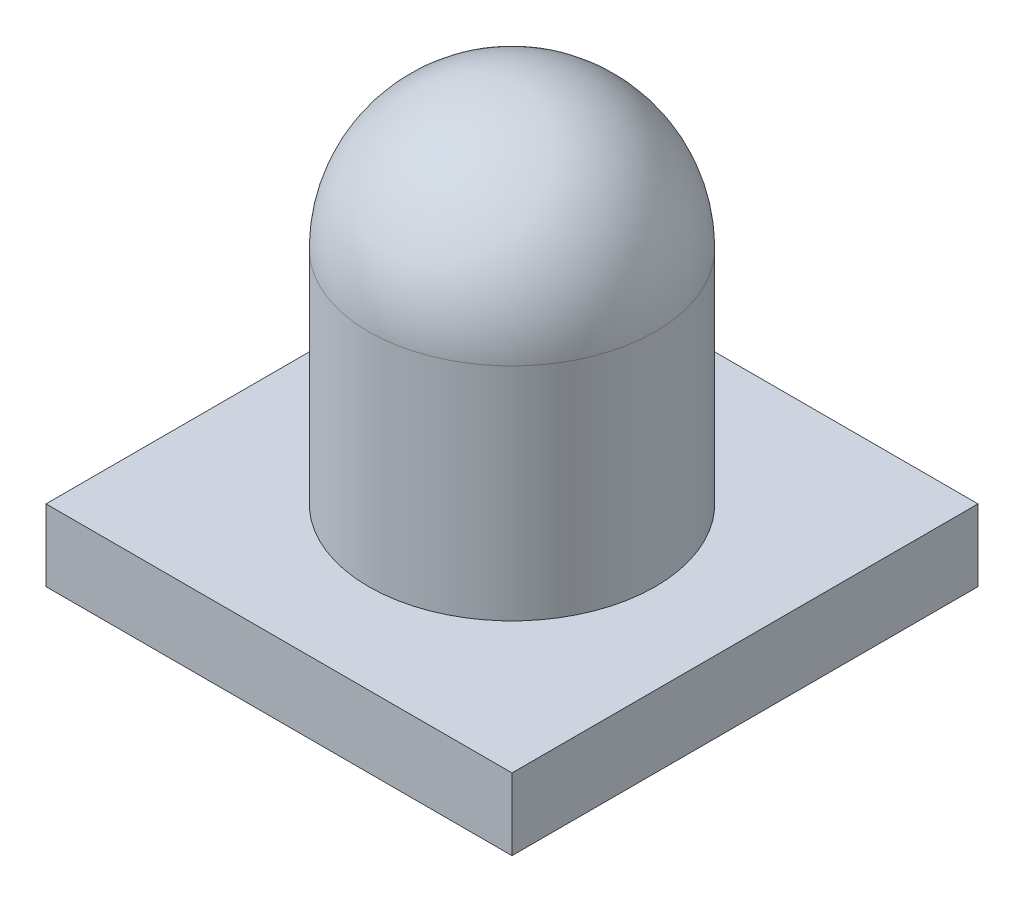
SolidWorks part; units mm, degrees
ref_plane "Front Plane" through (0, 0, 0) normal (0, 0, 1) x (1, 0, 0)
ref_plane "Top Plane" through (0, 0, 0) normal (0, 1, 0) x (1, 0, 0)
ref_plane "Right Plane" through (0, 0, 0) normal (1, 0, 0) x (0, 0, -1)
sketch "Sketch1" plane through (0, 0, 0) normal (0, 1, 0) x (1, 0, 0)
  line L1 (-32.5, -32.5) -> (32.5, -32.5)
  line L2 (-32.5, -32.5) -> (-32.5, 32.5)
  line L3 (-32.5, 32.5) -> (32.5, 32.5)
  line L4 (32.5, -32.5) -> (32.5, 32.5)
  line L5 (-32.5, -32.5) -> (32.5, 32.5) construction
  line L6 (-32.5, 32.5) -> (32.5, -32.5) construction
  point P0 (0, 0)
  dimension "D1" = 65
  dimension "D2" = 65
extrude "Boss-Extrude1" add sketch "Sketch1" along normal blind 10
sketch "Sketch2" plane through (0, 10, 0) normal (0, 1, 0) x (1, 0, 0)
  circle A0 centre (0, 0) radius 20
  dimension "D1" = 40
extrude "Boss-Extrude2" add sketch "Sketch2" along normal blind 50.8
fillet "Fillet1" radius 20 1 edges at (0, 60.8, 20)
sketch "Sketch3" plane through (0, 0, 0) normal (0, -1, 0) x (1, 0, 0)
  line L1 (-24, -18) -> (24, -18) construction
  line L2 (-24, -18) -> (-24, 18) construction
  line L3 (-24, 18) -> (24, 18) construction
  line L4 (24, -18) -> (24, 18) construction
  line L5 (-24, -18) -> (24, 18) construction
  line L6 (-24, 18) -> (24, -18) construction
  circle A0 centre (24, 18) radius 1.5
  circle A1 centre (-24, 18) radius 1.5
  circle A2 centre (-24, -18) radius 1.5
  circle A3 centre (24, -18) radius 1.5
  point P0 (0, 0)
  dimension "D3" = 3
  dimension "D4" = 3
  dimension "D5" = 3
  dimension "D6" = 3
  dimension "D1" = 48
  dimension "D2" = 36
extrude "Cut-Extrude1" cut sketch "Sketch3" against normal blind 5
